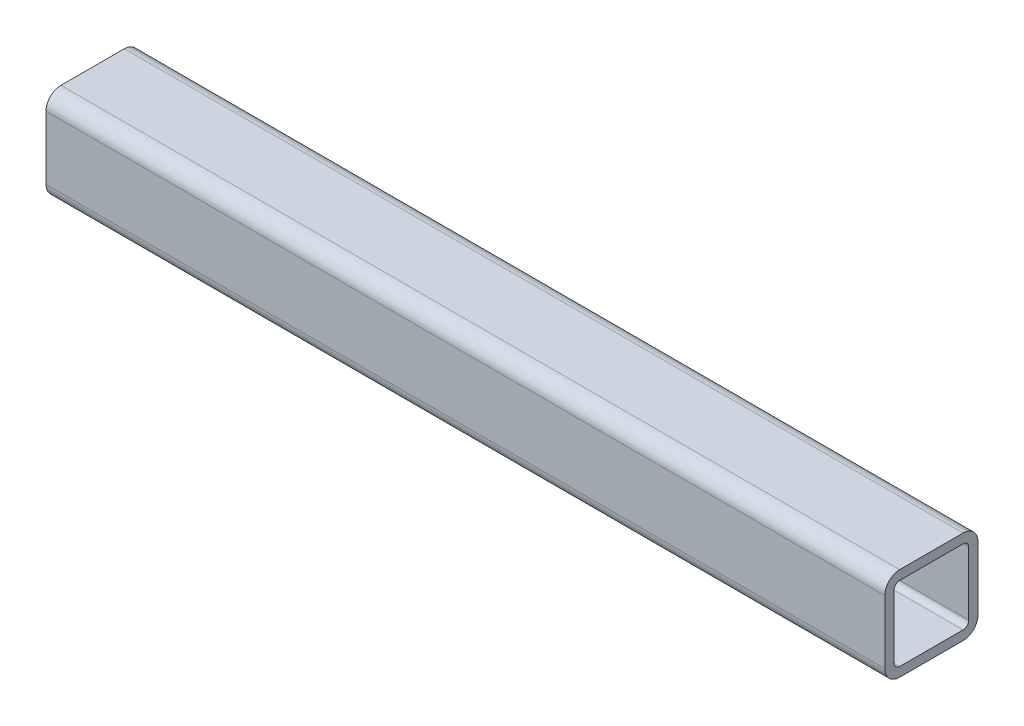
SolidWorks part; units mm, degrees
ref_plane "Front Plane" through (0, 0, 0) normal (0, 0, 1) x (1, 0, 0)
ref_plane "Top Plane" through (0, 0, 0) normal (0, 1, 0) x (1, 0, 0)
ref_plane "Right Plane" through (0, 0, 0) normal (1, 0, 0) x (0, 0, -1)
sketch "草图1" plane through (0, 0, 0) normal (0, 0, 1) x (1, 0, 0)
  line L0 (-88.4341, 0) -> (361.5659, 0)
  dimension "D1" = 450
other "Cold-formed square hollow section GB/T 6728-2002 50 X 50 X 4(1)"
ref_plane "Plane1" through (-88.4341, 0, 0) normal (1, 0, 0) x (0, 1, 0)
sketch "Sketch1" plane through (-88.4341, 0, 0) normal (1, 0, 0) x (0, 1, 0)
  line L0 (-17, -20) -> (17, -20)
  line L1 (-20, -17) -> (-20, 17)
  line L2 (17, 20) -> (-17, 20)
  line L3 (20, 17) -> (20, -17)
  line L4 (-17, -25) -> (17, -25)
  line L5 (-25, -17) -> (-25, 17)
  line L6 (17, 25) -> (-17, 25)
  line L7 (25, 17) -> (25, -17)
  arc A0 (25, 17) -> (17, 25) centre (17, 17) ccw
  arc A1 (17, -25) -> (25, -17) centre (17, -17) ccw
  arc A2 (-25, -17) -> (-17, -25) centre (-17, -17) ccw
  arc A3 (-17, 25) -> (-25, 17) centre (-17, 17) ccw
  arc A4 (-17, 20) -> (-20, 17) centre (-17, 17) ccw
  arc A5 (20, 17) -> (17, 20) centre (17, 17) ccw
  arc A6 (17, -20) -> (20, -17) centre (17, -17) ccw
  arc A7 (-20, -17) -> (-17, -20) centre (-17, -17) ccw
  point P0 (-25, 0)
  point P1 (25, 0)
  point P2 (0, 25)
  point P3 (0, -25)
  point P4 (0, 0)
  point P5 (-25, -25)
  point P6 (25, -25)
  point P7 (25, 25)
  point P8 (-25, 25)
  point P33 (0, 0)
  dimension "D1" = 8
  dimension "Thickness" = 5
  dimension "V_leg" = 50
